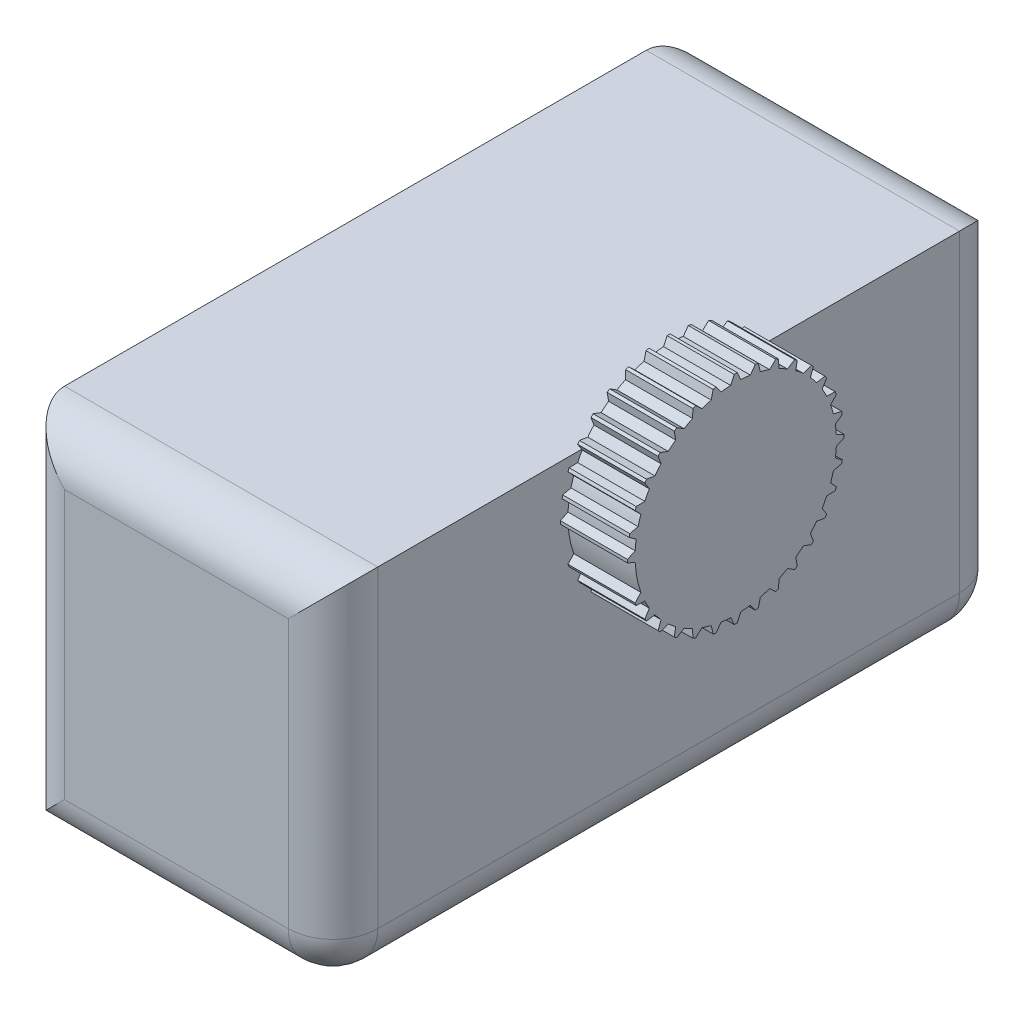
SolidWorks part; units mm, degrees
ref_plane "Front Plane" through (0, 0, 0) normal (0, 0, 1) x (1, 0, 0)
ref_plane "Top Plane" through (0, 0, 0) normal (0, 1, 0) x (1, 0, 0)
ref_plane "Right Plane" through (0, 0, 0) normal (1, 0, 0) x (0, 0, -1)
sketch "Sketch1" plane through (0, 0, 0) normal (0, 0, 1) x (1, 0, 0)
  line L1 (14, -16) -> (-14, -16)
  line L2 (14, -16) -> (14, 16)
  line L3 (14, 16) -> (-14, 16)
  line L4 (-14, -16) -> (-14, 16)
  line L5 (14, -16) -> (-14, 16) construction
  line L6 (14, 16) -> (-14, -16) construction
  point P0 (0, 0)
  dimension "D1" = 28
  dimension "D2" = 32
extrude "Boss-Extrude1" add sketch "Sketch1" along normal mid plane 60
sketch "Sketch2" plane through (14, 0, 0) normal (1, 0, 0) x (0, 0, -1)
  line L0 (0, 11.2939) -> (0, 19.2378) construction
  line L1 (-0.1371, 20.976) -> (0.1371, 20.976)
  line L2 (0.1371, 20.976) -> (0.4509, 20.2826)
  line L3 (-0.1371, 20.976) -> (-0.4509, 20.2826)
  line L4 (1.7544, 20.8167) -> (1.3114, 20.1978)
  line L5 (1.7544, 20.8167) -> (2.0234, 20.7632)
  line L6 (2.0234, 20.7632) -> (2.1958, 20.0219)
  line L7 (3.5785, 20.2914) -> (3.0233, 19.7709)
  line L8 (3.5785, 20.2914) -> (3.8319, 20.1865)
  line L9 (3.8319, 20.1865) -> (3.8564, 19.4258)
  line L10 (5.2651, 19.4204) -> (4.6189, 19.0182)
  line L11 (5.2651, 19.4204) -> (5.4931, 19.2681)
  line L12 (5.4931, 19.2681) -> (5.3688, 18.5172)
  line L13 (6.7493, 18.2371) -> (6.0371, 17.9687)
  line L14 (6.7493, 18.2371) -> (6.9432, 18.0432)
  line L15 (6.9432, 18.0432) -> (6.6748, 17.331)
  line L16 (7.9742, 16.787) -> (7.2233, 16.6626)
  line L17 (7.9742, 16.787) -> (8.1265, 16.559)
  line L18 (8.1265, 16.559) -> (7.7243, 15.9128)
  line L19 (8.8926, 15.1257) -> (8.1319, 15.1503)
  line L20 (8.8926, 15.1257) -> (8.9975, 14.8724)
  line L21 (8.9975, 14.8724) -> (8.477, 14.3171)
  line L22 (9.4693, 13.3172) -> (8.728, 13.4897)
  line L23 (9.4693, 13.3172) -> (9.5228, 13.0483)
  line L24 (9.5228, 13.0483) -> (8.9039, 12.6053)
  line L25 (9.6821, 11.431) -> (8.9887, 11.7448)
  line L26 (9.6821, 11.431) -> (9.6821, 11.1568)
  line L27 (9.6821, 11.1568) -> (8.9887, 10.843)
  line L28 (9.5228, 9.5395) -> (8.9039, 9.9825)
  line L29 (9.5228, 9.5395) -> (9.4693, 9.2705)
  line L30 (9.4693, 9.2705) -> (8.728, 9.0981)
  line L31 (8.9975, 7.7154) -> (8.477, 8.2706)
  line L32 (8.9975, 7.7154) -> (8.8926, 7.462)
  line L33 (8.8926, 7.462) -> (8.1319, 7.4375)
  line L34 (8.1265, 6.0288) -> (7.7243, 6.6749)
  line L35 (8.1265, 6.0288) -> (7.9742, 5.8008)
  line L36 (7.9742, 5.8008) -> (7.2233, 5.9251)
  line L37 (6.9432, 4.5446) -> (6.6748, 5.2567)
  line L38 (6.9432, 4.5446) -> (6.7493, 4.3507)
  line L39 (6.7493, 4.3507) -> (6.0371, 4.6191)
  line L40 (5.4931, 3.3197) -> (5.3688, 4.0706)
  line L41 (5.4931, 3.3197) -> (5.2651, 3.1674)
  line L42 (5.2651, 3.1674) -> (4.6189, 3.5696)
  line L43 (3.8319, 2.4013) -> (3.8564, 3.162)
  line L44 (3.8319, 2.4013) -> (3.5785, 2.2963)
  line L45 (3.5785, 2.2963) -> (3.0233, 2.8169)
  line L46 (2.0234, 1.8246) -> (2.1958, 2.5659)
  line L47 (2.0234, 1.8246) -> (1.7544, 1.7711)
  line L48 (1.7544, 1.7711) -> (1.3114, 2.3899)
  line L49 (0.1371, 1.6118) -> (0.4509, 2.3052)
  line L50 (0.1371, 1.6118) -> (-0.1371, 1.6118)
  line L51 (-0.1371, 1.6118) -> (-0.4509, 2.3052)
  line L52 (-1.7544, 1.7711) -> (-1.3114, 2.3899)
  line L53 (-1.7544, 1.7711) -> (-2.0234, 1.8246)
  line L54 (-2.0234, 1.8246) -> (-2.1958, 2.5659)
  line L55 (-3.5785, 2.2963) -> (-3.0233, 2.8169)
  line L56 (-3.5785, 2.2963) -> (-3.8319, 2.4013)
  line L57 (-3.8319, 2.4013) -> (-3.8564, 3.162)
  line L58 (-5.2651, 3.1674) -> (-4.6189, 3.5696)
  line L59 (-5.2651, 3.1674) -> (-5.4931, 3.3197)
  line L60 (-5.4931, 3.3197) -> (-5.3688, 4.0706)
  line L61 (-6.7493, 4.3507) -> (-6.0371, 4.6191)
  line L62 (-6.7493, 4.3507) -> (-6.9432, 4.5446)
  line L63 (-6.9432, 4.5446) -> (-6.6748, 5.2567)
  line L64 (-7.9742, 5.8008) -> (-7.2233, 5.9251)
  line L65 (-7.9742, 5.8008) -> (-8.1265, 6.0288)
  line L66 (-8.1265, 6.0288) -> (-7.7243, 6.6749)
  line L67 (-8.8926, 7.462) -> (-8.1319, 7.4375)
  line L68 (-8.8926, 7.462) -> (-8.9975, 7.7154)
  line L69 (-8.9975, 7.7154) -> (-8.477, 8.2706)
  line L70 (-9.4693, 9.2705) -> (-8.728, 9.0981)
  line L71 (-9.4693, 9.2705) -> (-9.5228, 9.5395)
  line L72 (-9.5228, 9.5395) -> (-8.9039, 9.9825)
  line L73 (-9.6821, 11.1568) -> (-8.9887, 10.843)
  line L74 (-9.6821, 11.1568) -> (-9.6821, 11.431)
  line L75 (-9.6821, 11.431) -> (-8.9887, 11.7448)
  line L76 (-9.5228, 13.0483) -> (-8.9039, 12.6053)
  line L77 (-9.5228, 13.0483) -> (-9.4693, 13.3172)
  line L78 (-9.4693, 13.3172) -> (-8.728, 13.4897)
  line L79 (-8.9975, 14.8724) -> (-8.477, 14.3171)
  line L80 (-8.9975, 14.8724) -> (-8.8926, 15.1257)
  line L81 (-8.8926, 15.1257) -> (-8.1319, 15.1503)
  line L82 (-8.1265, 16.559) -> (-7.7243, 15.9128)
  line L83 (-8.1265, 16.559) -> (-7.9742, 16.787)
  line L84 (-7.9742, 16.787) -> (-7.2233, 16.6626)
  line L85 (-6.9432, 18.0432) -> (-6.6748, 17.331)
  line L86 (-6.9432, 18.0432) -> (-6.7493, 18.2371)
  line L87 (-6.7493, 18.2371) -> (-6.0371, 17.9687)
  line L88 (-5.4931, 19.2681) -> (-5.3688, 18.5172)
  line L89 (-5.4931, 19.2681) -> (-5.2651, 19.4204)
  line L90 (-5.2651, 19.4204) -> (-4.6189, 19.0182)
  line L91 (-3.8319, 20.1865) -> (-3.8564, 19.4258)
  line L92 (-3.8319, 20.1865) -> (-3.5785, 20.2914)
  line L93 (-3.5785, 20.2914) -> (-3.0233, 19.7709)
  line L94 (-2.0234, 20.7632) -> (-2.1958, 20.0219)
  line L95 (-2.0234, 20.7632) -> (-1.7544, 20.8167)
  line L96 (-1.7544, 20.8167) -> (-1.3114, 20.1978)
  arc A0 (-0.4509, 20.2826) -> (-1.3114, 20.1978) centre (0, 11.2939) ccw
  arc A1 (-2.1958, 20.0219) -> (-3.0233, 19.7709) centre (0, 11.2939) ccw
  arc A2 (-3.8564, 19.4258) -> (-4.6189, 19.0182) centre (0, 11.2939) ccw
  arc A3 (-5.3688, 18.5172) -> (-6.0371, 17.9687) centre (0, 11.2939) ccw
  arc A4 (-6.6748, 17.331) -> (-7.2233, 16.6626) centre (0, 11.2939) ccw
  arc A5 (-7.7243, 15.9128) -> (-8.1319, 15.1503) centre (0, 11.2939) ccw
  arc A6 (-8.477, 14.3171) -> (-8.728, 13.4897) centre (0, 11.2939) ccw
  arc A7 (-8.9039, 12.6053) -> (-8.9887, 11.7448) centre (0, 11.2939) ccw
  arc A8 (-8.9887, 10.843) -> (-8.477, 8.2706) centre (0, 11.2939) ccw
  arc A9 (-8.1319, 7.4375) -> (-7.7243, 6.6749) centre (0, 11.2939) ccw
  arc A10 (-7.2233, 5.9251) -> (-6.6748, 5.2567) centre (0, 11.2939) ccw
  arc A11 (-6.0371, 4.6191) -> (-5.3688, 4.0706) centre (0, 11.2939) ccw
  arc A12 (-4.6189, 3.5696) -> (-3.8564, 3.162) centre (0, 11.2939) ccw
  arc A13 (-3.0233, 2.8169) -> (-2.1958, 2.5659) centre (0, 11.2939) ccw
  arc A14 (-1.3114, 2.3899) -> (-0.4509, 2.3052) centre (0, 11.2939) ccw
  arc A15 (0.4509, 2.3052) -> (1.3114, 2.3899) centre (0, 11.2939) ccw
  arc A16 (2.1958, 2.5659) -> (3.0233, 2.8169) centre (0, 11.2939) ccw
  arc A17 (1.3114, 20.1978) -> (0.4509, 20.2826) centre (0, 11.2939) ccw
  arc A18 (3.0233, 19.7709) -> (2.1958, 20.0219) centre (0, 11.2939) ccw
  arc A19 (4.6189, 19.0182) -> (3.8564, 19.4258) centre (0, 11.2939) ccw
  arc A20 (6.0371, 17.9687) -> (5.3688, 18.5172) centre (0, 11.2939) ccw
  arc A21 (7.2233, 16.6626) -> (6.6748, 17.331) centre (0, 11.2939) ccw
  arc A22 (8.1319, 15.1503) -> (7.7243, 15.9128) centre (0, 11.2939) ccw
  arc A23 (8.728, 13.4897) -> (8.477, 14.3171) centre (0, 11.2939) ccw
  arc A24 (8.9887, 11.7448) -> (8.9039, 12.6053) centre (0, 11.2939) ccw
  arc A25 (8.9039, 9.9825) -> (8.9887, 10.843) centre (0, 11.2939) ccw
  arc A26 (8.477, 8.2706) -> (8.728, 9.0981) centre (0, 11.2939) ccw
  arc A27 (7.7243, 6.6749) -> (8.1319, 7.4375) centre (0, 11.2939) ccw
  arc A28 (6.6748, 5.2567) -> (7.2233, 5.9251) centre (0, 11.2939) ccw
  arc A29 (5.3688, 4.0706) -> (6.0371, 4.6191) centre (0, 11.2939) ccw
  arc A30 (3.8564, 3.162) -> (4.6189, 3.5696) centre (0, 11.2939) ccw
  point P134 (0, 11.2939)
  dimension "D1" = 18
  dimension "D2" = 32
extrude "Boss-Extrude3" add sketch "Sketch2" along normal blind 6
fillet "Fillet1" radius 4 9 edges at (0, -16, -30) (14, 0, -30) (0, 16, -30) (-14, 0, -30) (0, 16, 30) (14, 0, 30) (0, -16, 30) (-14, 0, 30) (14, -16, 0)
sketch "Sketch4" plane through (0, -16, 0) normal (0, -1, 0) x (1, 0, 0)
  line L0 (10, -30) -> (-10, -30) construction
  circle A0 centre (-2, 10) radius 3.7665
  circle A1 centre (-2, -10) radius 3.7238
  point P0 (-2, 10)
  point P2 (-2, -10)
  dimension "D1" = 20
  dimension "D2" = 20
hole_wizard "Tap Drill for M8 Tap1" positions "Sketch4" profile "Sketch5" hole size "M8" standard "GB"
sketch "Sketch5" plane through (-2, -16, 10) normal (1, 0, 0) x (0, 0, -1)
  line L0 (0, 0) -> (0, 7.0429)
  line L1 (0, 7.0429) -> (3.4, 5)
  line L2 (3.4, 5) -> (3.4, 0)
  line L5 (3.4, 0) -> (0, 0)
  line L10 (0, 7.0429) -> (-3.4, 5) construction
  line L11 (0, -6.35) -> (0, 107.95) construction
  dimension "孔直径" = 6.8
  dimension "孔深度" = 5
  dimension "导头角度" = 118
